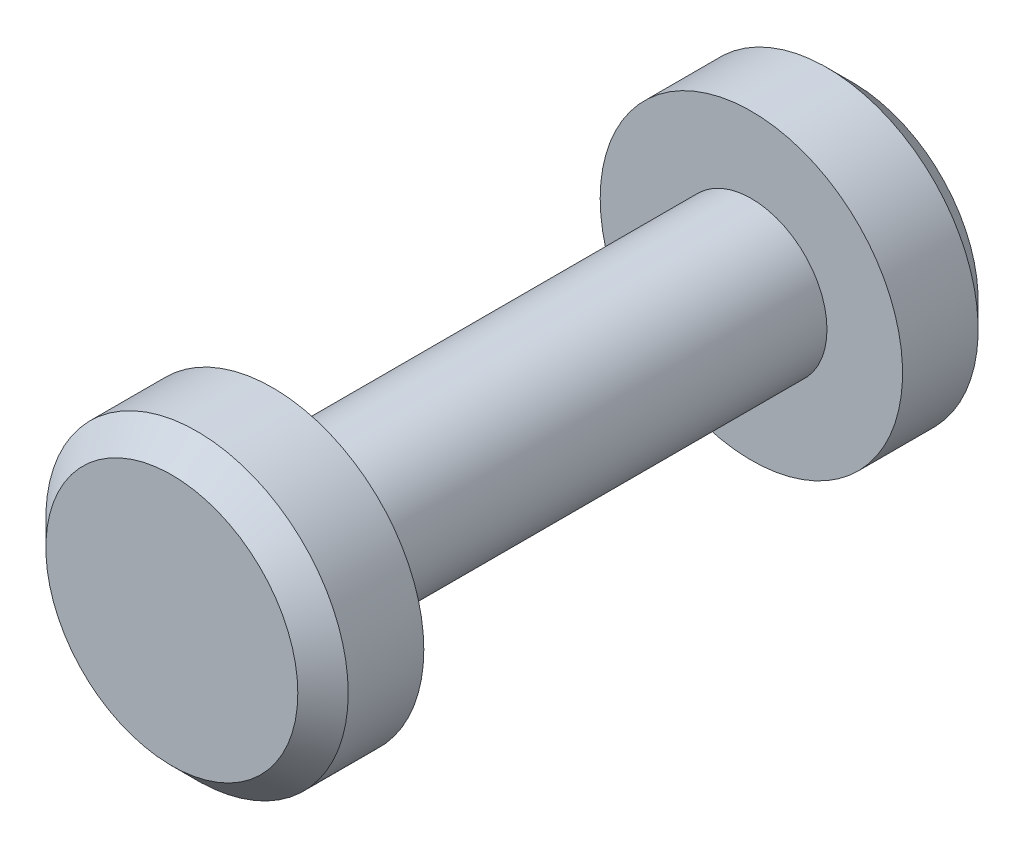
SolidWorks part; units mm, degrees
ref_plane "前视基准面" through (0, 0, 0) normal (0, 0, 1) x (1, 0, 0)
ref_plane "上视基准面" through (0, 0, 0) normal (0, 1, 0) x (1, 0, 0)
ref_plane "右视基准面" through (0, 0, 0) normal (1, 0, 0) x (0, 0, -1)
sketch "草图1" plane through (0, 0, 0) normal (0, 0, 1) x (1, 0, 0)
  circle A0 centre (0, 0) radius 3
extrude "凸台-拉伸1" add sketch "草图1" along normal blind 19
sketch "草图2" plane through (0, 0, 19) normal (0, 0, 1) x (1, 0, 0)
  circle A0 centre (0, 0) radius 6
extrude "凸台-拉伸2" add sketch "草图2" along normal blind 4
chamfer "倒角1" distance 1 angle 45 1 edges at (6, 0, 23)
sketch "草图3" plane through (0, 0, 0) normal (0, 0, -1) x (-1, 0, 0)
  circle A0 centre (0, 0) radius 6
extrude "凸台-拉伸3" add sketch "草图3" along normal blind 4
chamfer "倒角2" distance 1 angle 45 1 edges at (-6, 0, -4)
